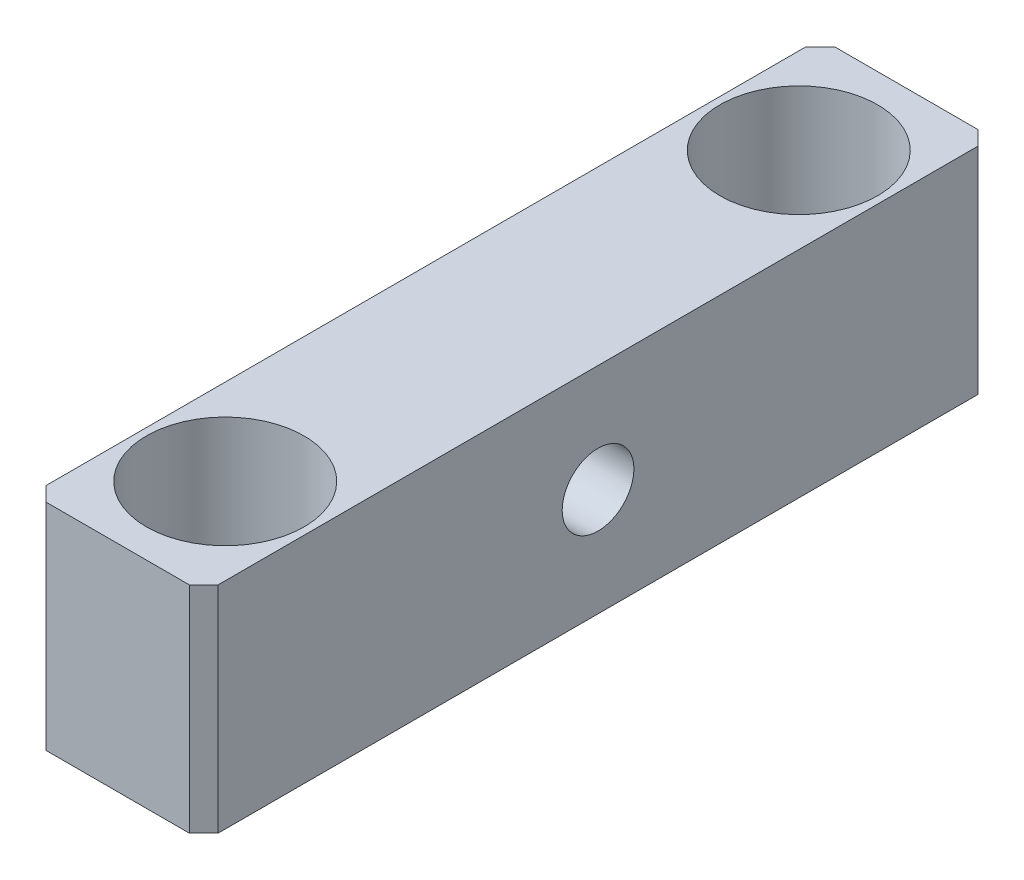
SolidWorks part; units mm, degrees
material "S45C"
ref_plane "前视基准面" through (0, 0, 0) normal (0, 0, 1) x (1, 0, 0)
ref_plane "上视基准面" through (0, 0, 0) normal (0, 1, 0) x (1, 0, 0)
ref_plane "右视基准面" through (0, 0, 0) normal (1, 0, 0) x (0, 0, -1)
sketch "草图1" plane through (0, 0, 0) normal (0, 1, 0) x (1, 0, 0)
  line L1 (-6, -27.5) -> (6, -27.5)
  line L2 (-6, -27.5) -> (-6, 27.5)
  line L3 (-6, 27.5) -> (6, 27.5)
  line L4 (6, -27.5) -> (6, 27.5)
  line L5 (-6, -27.5) -> (6, 27.5) construction
  line L6 (-6, 27.5) -> (6, -27.5) construction
  point P0 (0, 0)
  dimension "D1" = 12
  dimension "D2" = 55
extrude "凸台-拉伸1" add sketch "草图1" along normal mid plane 15
chamfer "倒角1" distance 1 angle 45 4 edges at (6, 0, -27.5) (-6, 0, -27.5) (6, 0, 27.5) (-6, 0, 27.5)
sketch "草图2" plane through (0, 7.5, 0) normal (0, 1, 0) x (1, 0, 0)
  line L0 (-6, 0) -> (10.5286, 0) construction
  line L1 (-6, 26.5) -> (-6, -26.5) construction
  point P0 (0, 20)
  point P2 (0, -20)
  dimension "D1" = 40
hole_wizard "M6 六角圆柱头螺钉的柱形沉头孔1" positions "草图2" profile "草图3" counterbore size "M6" standard "GB" end condition up to next
sketch "草图3" plane through (0, 7.5, -20) normal (1, 0, 0) x (0, 0, 1)
  line L0 (0, 0) -> (0, 15)
  line L1 (0, 15) -> (3.3, 15)
  line L3 (3.3, 15) -> (3.3, 8)
  line L4 (3.3, 8) -> (5.5, 8)
  line L5 (5.5, 8) -> (5.5, 0)
  line L7 (5.5, 0) -> (0, 0)
  line L11 (0, -6.35) -> (0, 107.95) construction
  dimension "通孔孔直径" = 6.6
  dimension "通孔孔深度" = 15
  dimension "柱形沉头孔直径" = 11
  dimension "柱形沉头孔深度" = 8
sketch "草图4" plane through (-6, 0, 0) normal (-1, 0, 0) x (0, 0, 1)
  point P0 (0, 0)
hole_wizard "M6 螺纹孔1" positions "草图4" profile "草图5" tap size "M6" standard "GB" end condition up to next
sketch "草图5" plane through (-6, 0, 0) normal (0, 1, 0) x (0, 0, 1)
  line L0 (0, 0) -> (0, 12)
  line L1 (0, 12) -> (2.5, 12)
  line L2 (2.5, 12) -> (2.5, 0)
  line L5 (2.5, 0) -> (0, 0)
  line L11 (0, -6.35) -> (0, 107.95) construction
  dimension "通孔螺纹孔钻头直径" = 5
  dimension "通孔螺纹孔钻头深度" = 12
cosmetic thread "孔螺纹线1" parameters "D2"=6
